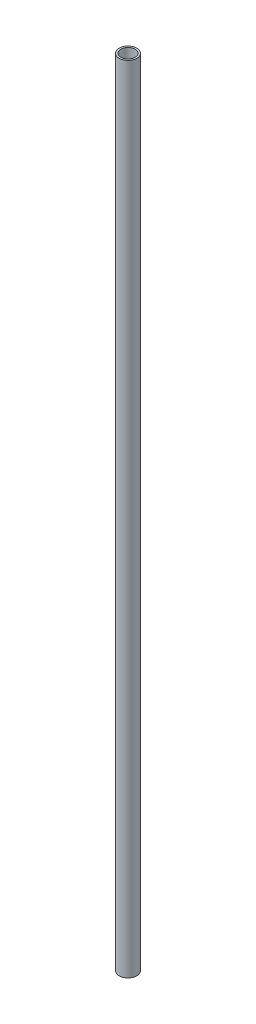
from build123d import *

# Parameters (mm, degrees)
SWEEP_THIN1_PROFILE_R   = 10
SWEEP_THIN1_PROFILE_R_2 = 8


with BuildPart() as part:
    # Sweep-Thin1: sweep along a path in Sketch1
    with BuildLine(Plane.XY) as sweep_thin1_path:
        Line((0, 0), (0, 900))
    # Sweep-Thin1 profile (on start of the path) → Sweep-Thin1 (sweep)
    with BuildSketch(Plane.ZX):
        Circle(SWEEP_THIN1_PROFILE_R)
        Circle(SWEEP_THIN1_PROFILE_R_2, mode=Mode.SUBTRACT)
    sweep(path=sweep_thin1_path.line)


solid = part.part
